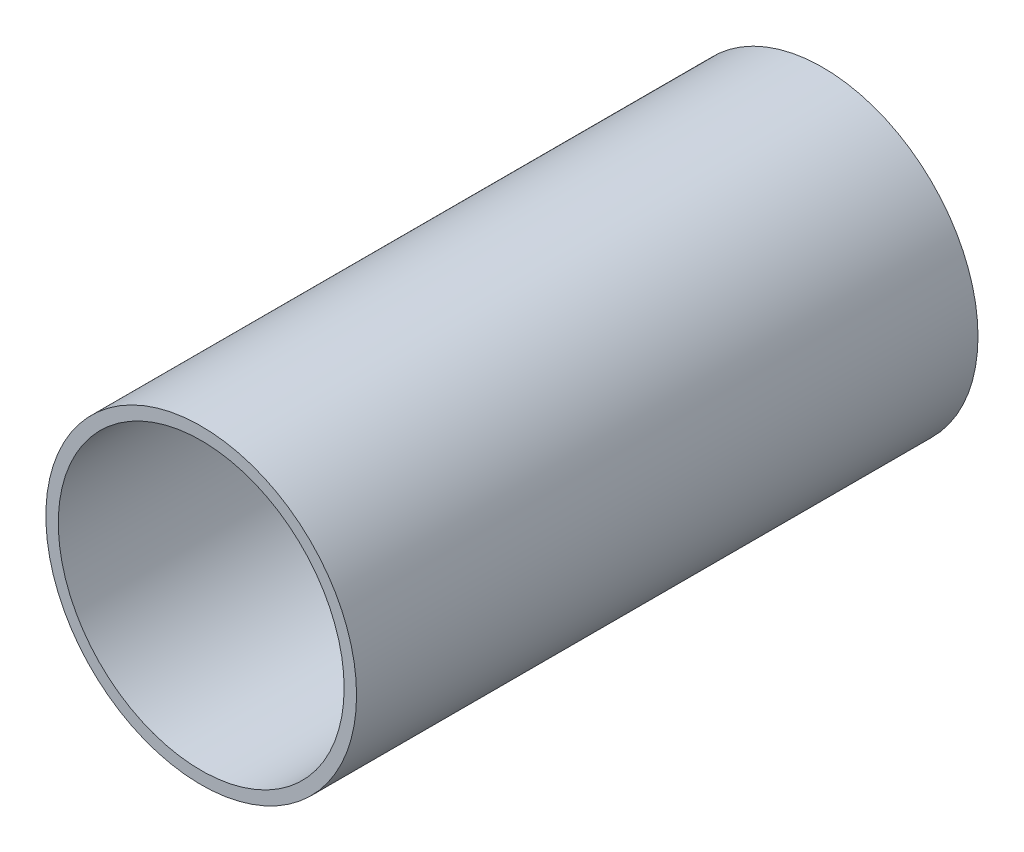
SolidWorks part; units mm, degrees
ref_plane "Front Plane" through (0, 0, 0) normal (0, 0, 1) x (1, 0, 0)
ref_plane "Top Plane" through (0, 0, 0) normal (0, 1, 0) x (1, 0, 0)
ref_plane "Right Plane" through (0, 0, 0) normal (1, 0, 0) x (0, 0, -1)
sketch "Sketch1" plane through (0, 0, 0) normal (0, 0, 1) x (1, 0, 0)
  circle A0 centre (0, 0) radius 25
  circle A1 centre (0, 0) radius 23
  dimension "D1" = 50
  dimension "D2" = 2
extrude "Boss-Extrude1" add sketch "Sketch1" along normal blind 100
